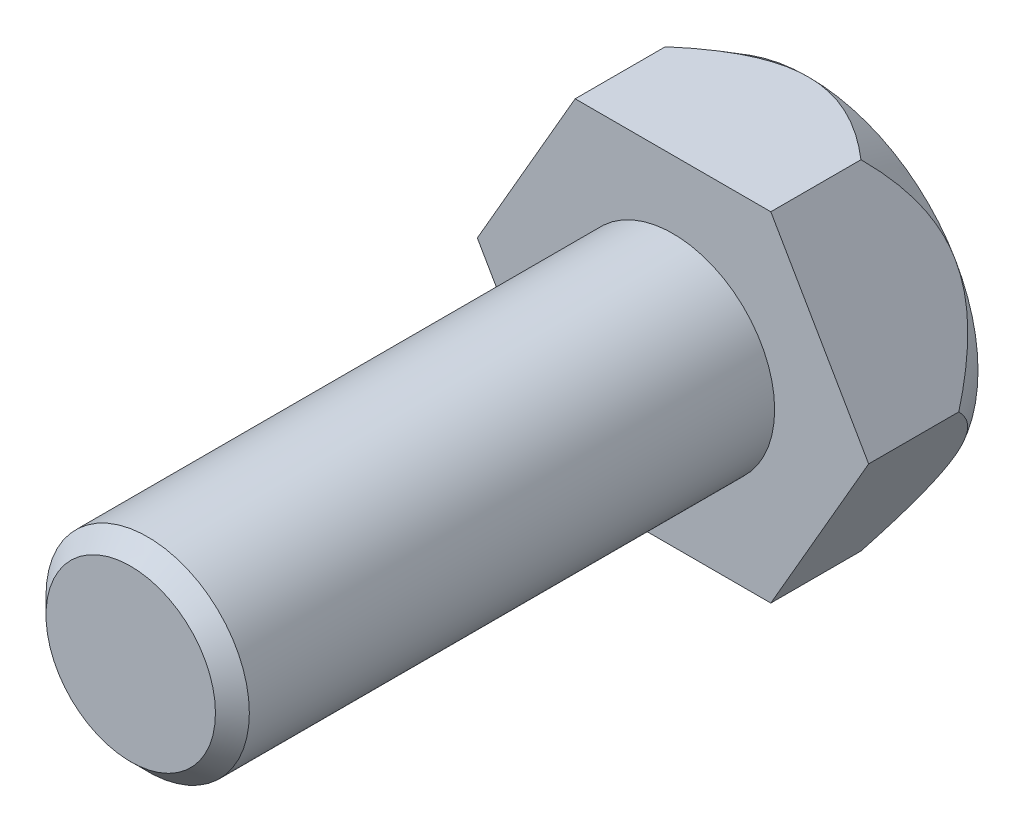
SolidWorks part; units mm, degrees
ref_plane "Front Plane" through (0, 0, 0) normal (0, 0, 1) x (1, 0, 0)
ref_plane "Top Plane" through (0, 0, 0) normal (0, 1, 0) x (1, 0, 0)
ref_plane "Right Plane" through (0, 0, 0) normal (1, 0, 0) x (0, 0, -1)
other "Configuration Table"
sketch "Sketch1" plane through (0, 0, 0) normal (0, 0, 1) x (1, 0, 0)
  line L1 (2.8868, 5) -> (-2.8868, 5)
  line L2 (-2.8868, 5) -> (-5.7735, 0)
  line L3 (-5.7735, 0) -> (-2.8868, -5)
  line L4 (-2.8868, -5) -> (2.8868, -5)
  line L5 (2.8868, -5) -> (5.7735, 0)
  line L6 (5.7735, 0) -> (2.8868, 5)
  circle A2 centre (0, 0) radius 5 construction
  dimension "D1" = 10
extrude "Boss-Extrude1" add sketch "Sketch1" along normal blind 4
sketch "Sketch2" plane through (0, 0, 0) normal (0, 0, -1) x (-1, 0, 0)
  line L0 (-5.7735, 0) -> (-2.8868, 5) construction
  circle A0 centre (0, 0) radius 5
extrude "Cut-Extrude1" cut sketch "Sketch2" against normal blind 4 draft 30 flip side to cut
sketch "Sketch3" plane through (0, 0, 4) normal (0, 0, 1) x (1, 0, 0)
  circle A0 centre (0, 0) radius 3
  dimension "D1" = 6
extrude "Boss-Extrude2" add sketch "Sketch3" along normal blind 16
cosmetic thread "Cosmetic Thread1" parameters "D2"=4.917
chamfer "Chamfer1" distance 0.5 angle 45 1 edges at (3, 0, 20)
